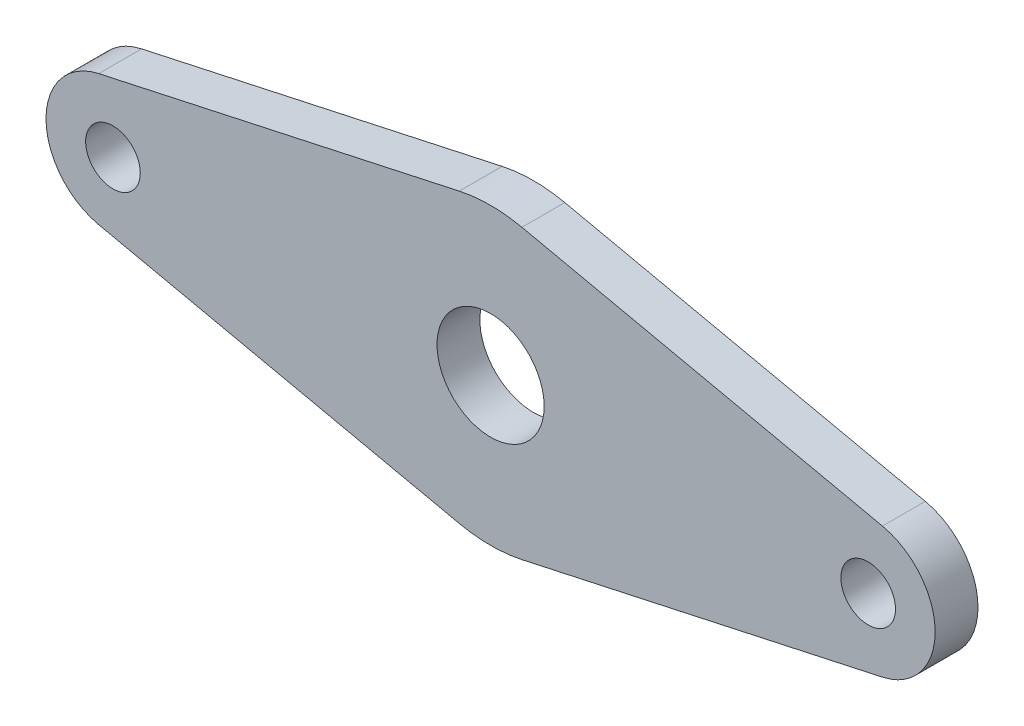
from build123d import *

# Parameters (mm, degrees)
EXTRUDE_1_DEPTH         = 8
HOLE_WIZARD_M12_1_D     = 10.2
HOLE_WIZARD_M12_1_DEPTH = 29.25
HOLE_WIZARD_M12_1_TIP   = 3.064389157
SKETCH_5_R              = 10
CUT_EXTRUDE_1_DEPTH     = 8


with BuildPart() as part:
    # 草图1 → 凸台-拉伸1 (new body)
    with BuildSketch(Plane.XY):
        with BuildLine():
            Line((-73.159574468, 12.213789897), (-5.85106383, 26.870337773))
            ThreePointArc((-5.85106383, 26.870337773), (0, 27.5), (5.85106383, 26.870337773))
            Line((5.85106383, 26.870337773), (73.159574468, 12.213789897))
            ThreePointArc((73.159574468, 12.213789897), (83, 0), (73.159574468, -12.213789897))
            Line((73.159574468, -12.213789897), (5.85106383, -26.870337773))
            ThreePointArc((5.85106383, -26.870337773), (0, -27.5), (-5.85106383, -26.870337773))
            Line((-5.85106383, -26.870337773), (-73.159574468, -12.213789897))
            ThreePointArc((-73.159574468, -12.213789897), (-83, 0), (-73.159574468, 12.213789897))
        make_face()
    extrude(amount=EXTRUDE_1_DEPTH)

    # M12 螺纹孔1
    with Locations(Plane.XY.offset(8)):
        with Locations((-70.5, 0), (70.5, 0)):
            Hole(HOLE_WIZARD_M12_1_D / 2, depth=HOLE_WIZARD_M12_1_DEPTH)
            with Locations((0, 0, -(HOLE_WIZARD_M12_1_DEPTH + HOLE_WIZARD_M12_1_TIP / 2))):  # 118° drill point
                Cone(0, HOLE_WIZARD_M12_1_D / 2, HOLE_WIZARD_M12_1_TIP, mode=Mode.SUBTRACT)

    # 草图5 → 切除-拉伸1 (cut)
    with BuildSketch(Plane.XY.offset(8)):
        Circle(SKETCH_5_R)
    extrude(amount=-CUT_EXTRUDE_1_DEPTH, mode=Mode.SUBTRACT)


solid = part.part
